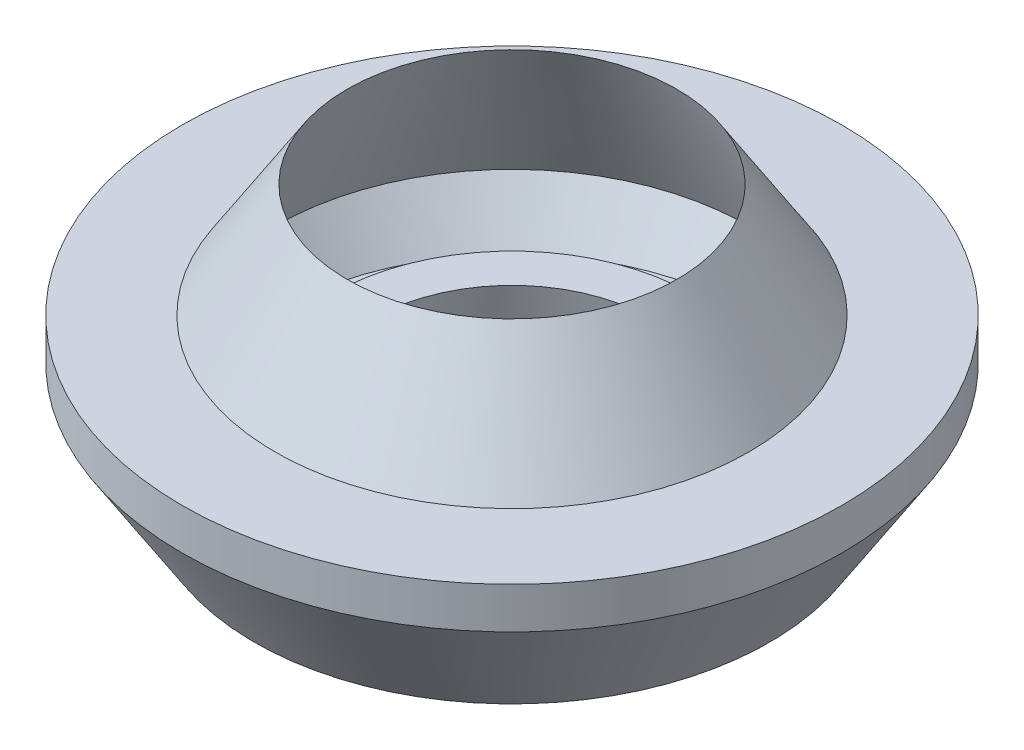
from build123d import *


with BuildPart() as part:
    # 草图1 → 旋转1 (revolve)
    with BuildSketch(Plane.XY, mode=Mode.PRIVATE) as revolve_1_sk:
        Polygon((16, 26), (23, 15), (32, 15), (32, 11), (25, 0), (15, 0), (13.45, 8), (17.524386457, 8), (18.299386457, 4), (22.804216433, 4), (27.258761887, 11), (22.994614872, 11), align=None)
    revolve(revolve_1_sk.sketch.rotate(Axis((0, 12.915252942, 0), (0, -1, 0)), 180), axis=Axis((0, 12.915252942, 0), (0, -1, 0)))


solid = part.part
